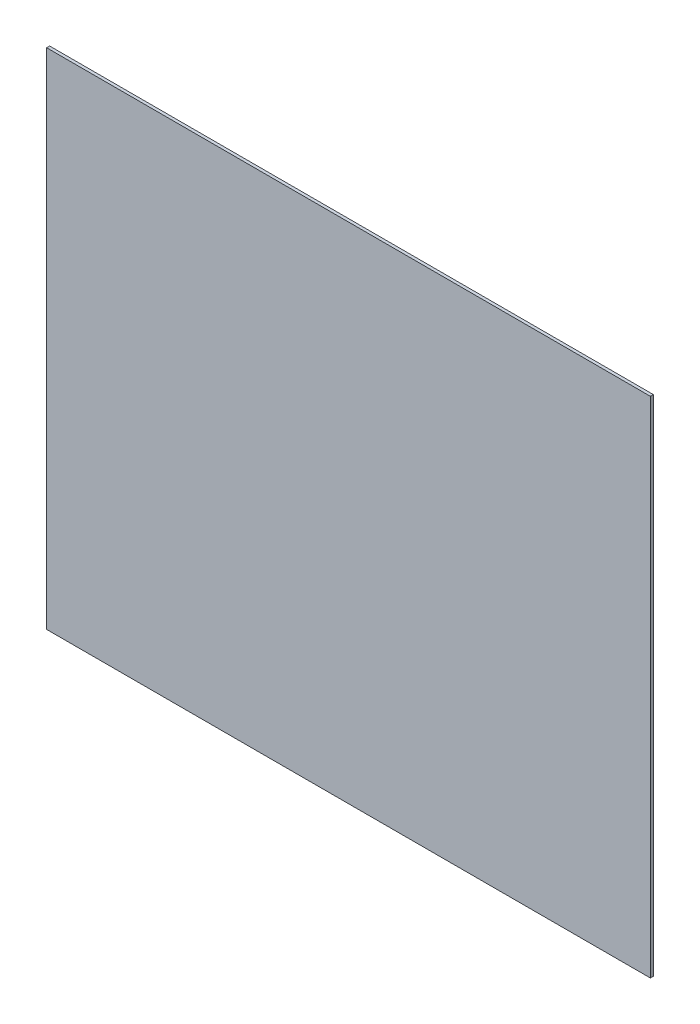
from build123d import *

# Parameters (mm, degrees)
SKETCH_1_W      = 1009
SKETCH_1_H      = 842
EXTRUDE_1_DEPTH = 5


with BuildPart() as part:
    # 草图1 → 凸台-拉伸1 (new body)
    with BuildSketch(Plane.XY):
        Rectangle(SKETCH_1_W, SKETCH_1_H)
    extrude(amount=EXTRUDE_1_DEPTH)


solid = part.part
